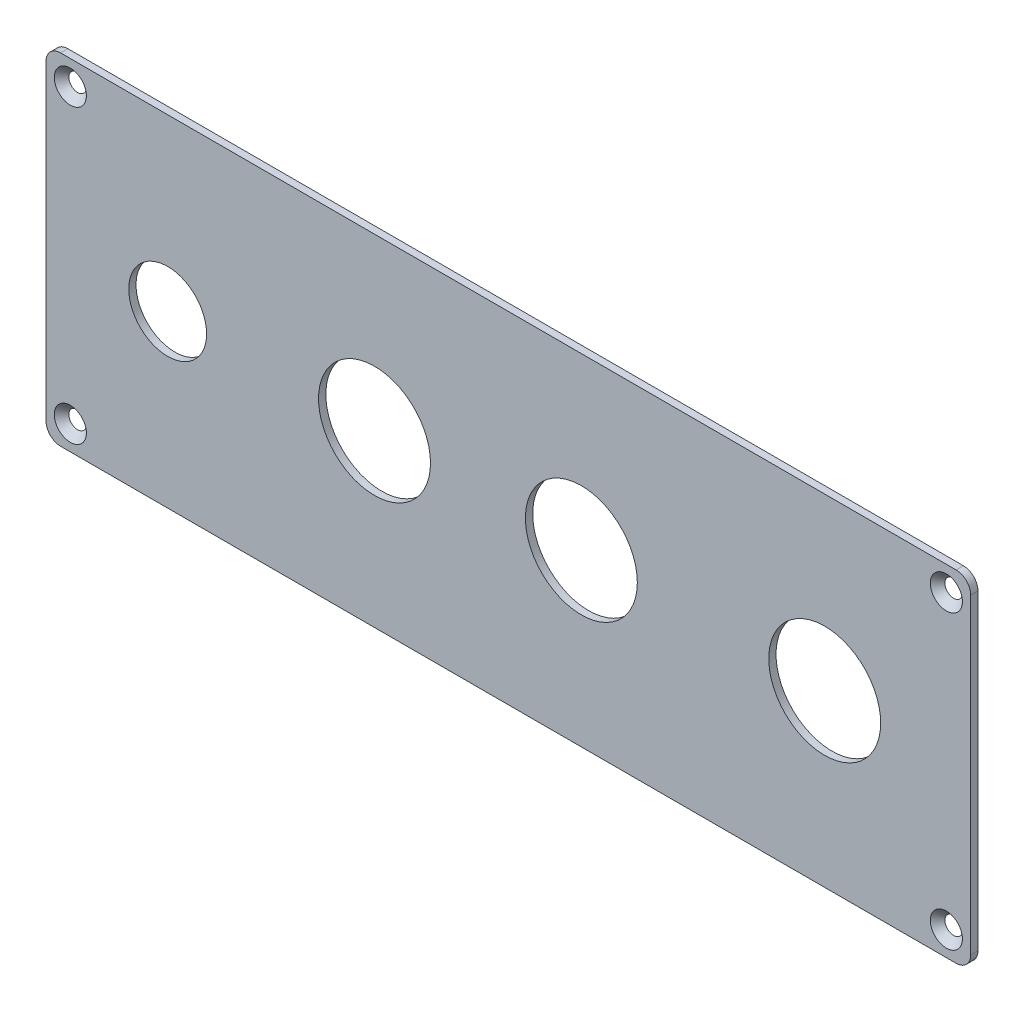
from build123d import *

# Parameters (mm, degrees)
SKETCH_1_W               = 190
SKETCH_1_H               = 70
EXTRUDE_1_DEPTH          = 1.5
FILLET_1_R               = 3
SKETCH_2_R               = 11.5
SKETCH_2_R_2             = 8
CUT_EXTRUDE_1_DEPTH      = 1.5
HOLE_WIZARD_1_AT_2_COUNT = 2
HOLE_WIZARD_1_AT_2_PITCH = 60
HOLE_WIZARD_1_AT_3_COUNT = 2
HOLE_WIZARD_1_AT_3_PITCH = 189.73665961
HOLE_WIZARD_1_AT_4_COUNT = 2
HOLE_WIZARD_1_AT_4_PITCH = 180


with BuildPart() as part:
    # 草图1 → 凸台-拉伸1 (new body)
    with BuildSketch(Plane.XY):
        Rectangle(SKETCH_1_W, SKETCH_1_H)
    extrude(amount=EXTRUDE_1_DEPTH)

    # 圆角1
    fillet_1_edges = [part.edges().sort_by_distance(p)[0] for p in [
        (95, -35, 0.75),
        (-95, -35, 0.75),
        (-95, 35, 0.75),
        (95, 35, 0.75),
    ]]
    fillet(fillet_1_edges, radius=FILLET_1_R)

    # 草图2 → 切除-拉伸1 (cut)
    with BuildSketch(Plane.XY.offset(1.5)):
        with Locations((15, 0)):
            Circle(SKETCH_2_R)
        with Locations((-27.5, 0)):
            Circle(SKETCH_2_R)
        with Locations((65, 0)):
            Circle(SKETCH_2_R)
        with Locations((-70, 0)):
            Circle(SKETCH_2_R_2)
    extrude(amount=-CUT_EXTRUDE_1_DEPTH, mode=Mode.SUBTRACT)

    # 草图4 → 打孔尺寸根据十字槽半沉头木螺钉的类型1 (revolve, cut)
    with BuildSketch(Plane(origin=(-90, 30, 1.5), x_dir=(0, -1, 0), z_dir=(1, 0, 0))):
        Polygon((0, 0), (0, 1.5), (1.7, 1.5), (1.7, 1.6), (3.3, 0), align=None)
    hole_wizard_1 = revolve(axis=Axis((-90, 30, 7.85), (0, 0, -1)), mode=Mode.SUBTRACT)

    # 打孔尺寸根据十字槽半沉头木螺钉的类型1 at 2: 打孔尺寸根据十字槽半沉头木螺钉的类型1 ×2
    with Locations(*[(0, -i * HOLE_WIZARD_1_AT_2_PITCH, 0) for i in range(1, HOLE_WIZARD_1_AT_2_COUNT)]):
        add(hole_wizard_1, mode=Mode.SUBTRACT)

    # 打孔尺寸根据十字槽半沉头木螺钉的类型1 at 3: 打孔尺寸根据十字槽半沉头木螺钉的类型1 ×2
    with Locations(*[Vector(0.9486832980505139, -0.3162277660168379, 0) * (i * HOLE_WIZARD_1_AT_3_PITCH) for i in range(1, HOLE_WIZARD_1_AT_3_COUNT)]):
        add(hole_wizard_1, mode=Mode.SUBTRACT)

    # 打孔尺寸根据十字槽半沉头木螺钉的类型1 at 4: 打孔尺寸根据十字槽半沉头木螺钉的类型1 ×2
    with Locations(*[(i * HOLE_WIZARD_1_AT_4_PITCH, 0, 0) for i in range(1, HOLE_WIZARD_1_AT_4_COUNT)]):
        add(hole_wizard_1, mode=Mode.SUBTRACT)


solid = part.part
